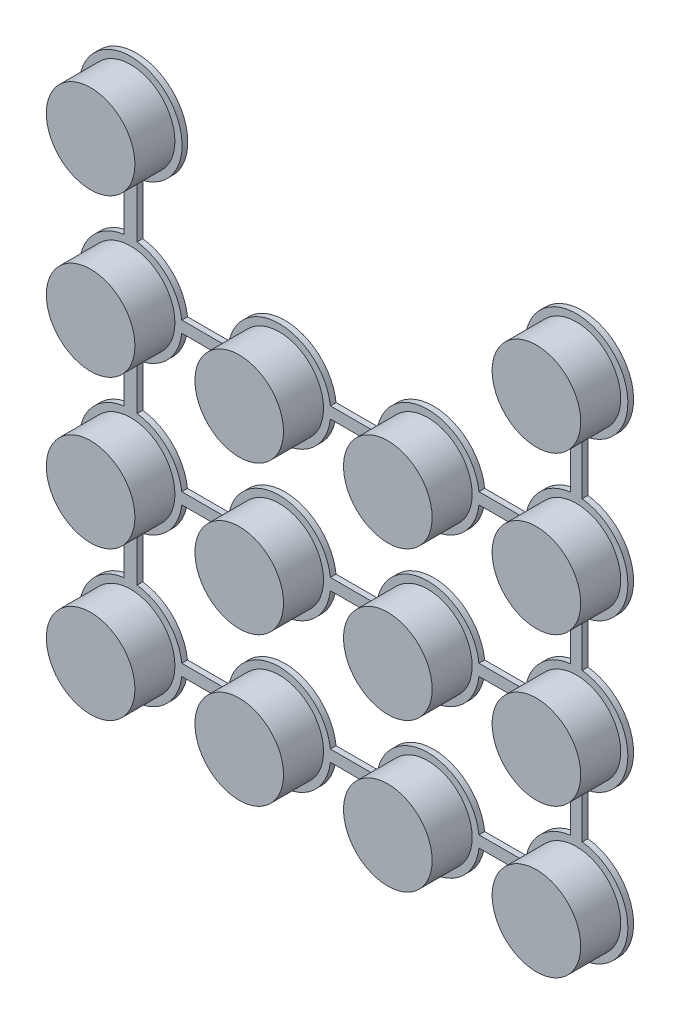
SolidWorks part; units mm, degrees
ref_plane "Front Plane" through (0, 0, 0) normal (0, 0, 1) x (1, 0, 0)
ref_plane "Top Plane" through (0, 0, 0) normal (0, 1, 0) x (1, 0, 0)
ref_plane "Right Plane" through (0, 0, 0) normal (1, 0, 0) x (0, 0, -1)
other "Configuration Table"
sketch "Sketch1" plane through (0, 0, 0) normal (0, 0, 1) x (1, 0, 0)
  line L0 (0, 0) -> (0, 200) construction
  line L9 (-37.875, 23) -> (-30, 23) construction
  line L10 (39, 48) -> (39, 58) construction
  line L15 (-37.875, 23) -> (-30, 23) construction
  line L16 (-40.125, 93.5706) -> (-40.125, 83.9294)
  line L17 (-37.875, 93.5706) -> (-37.875, 83.9294)
  line L18 (-30.0557, 76) -> (-21.9443, 76)
  line L19 (-30.0557, 74) -> (-21.9443, 74)
  line L20 (-30.0557, 50) -> (-21.9443, 50)
  line L21 (40, 23) -> (40, 102.5) construction
  line L22 (-30.0557, 48) -> (-21.9443, 48)
  line L23 (-30.0557, 22) -> (-21.9443, 22)
  line L24 (-30.0557, 24) -> (-21.9443, 24)
  line L25 (38, 31.9443) -> (38, 40.0557)
  line L26 (40, 31.9443) -> (40, 40.0557)
  line L27 (39, 23) -> (39, 102.5) construction
  line L28 (38, 23) -> (38, 102.5) construction
  line L29 (38, 83.9443) -> (38, 93.5557)
  line L30 (40, 83.9443) -> (40, 93.5557)
  line L31 (39, 74) -> (39, 76) construction
  line L32 (21.9443, 74) -> (30.0557, 74)
  line L33 (21.9443, 76) -> (30.0557, 76)
  line L35 (-5, 75) -> (0, 75) construction
  line L37 (-4.0557, 74) -> (4.0557, 74)
  line L39 (-4.0557, 76) -> (4.0557, 76)
  line L40 (-4.0557, 48) -> (4.0557, 48)
  line L44 (-4.0557, 50) -> (4.0557, 50)
  line L46 (-37.875, 66.0706) -> (-37.875, 57.9294)
  line L47 (-37.875, 40.0706) -> (-37.875, 31.9294)
  line L48 (-39, 22) -> (39, 22) construction
  line L50 (-40.125, 66.0706) -> (-40.125, 57.9294)
  line L51 (-40.125, 40.0706) -> (-40.125, 31.9294)
  line L52 (-39, 23) -> (39, 23) construction
  line L53 (-39, 24) -> (39, 24) construction
  line L55 (-4.0557, 24) -> (4.0557, 24)
  line L56 (-4.0557, 22) -> (4.0557, 22)
  line L57 (21.9443, 24) -> (30.0557, 24)
  line L58 (21.9443, 22) -> (30.0557, 22)
  line L59 (21.9443, 48) -> (30.0557, 48)
  line L60 (40, 57.9443) -> (40, 66.0557)
  line L61 (38, 57.9443) -> (38, 66.0557)
  line L62 (21.9443, 50) -> (30.0557, 50)
  arc A0 (-21.9443, 22) -> (-4.0557, 22) centre (-13, 23) ccw
  arc A1 (-40.125, 31.9294) -> (-30.0557, 22) centre (-39, 23) ccw
  arc A2 (-40.125, 57.9294) -> (-40.125, 40.0706) centre (-39, 49) ccw
  arc A3 (-4.0557, 50) -> (-21.9443, 50) centre (-13, 49) ccw
  arc A4 (-40.125, 83.9294) -> (-40.125, 66.0706) centre (-39, 75) ccw
  arc A5 (-4.0557, 76) -> (-21.9443, 76) centre (-13, 75) ccw
  arc A8 (-37.875, 93.5706) -> (-40.125, 93.5706) centre (-39, 102.5) ccw
  arc A10 (21.9443, 74) -> (4.0557, 74) centre (13, 75) cw
  arc A11 (40, 83.9443) -> (40, 66.0557) centre (39, 75) cw
  arc A12 (21.9443, 48) -> (4.0557, 48) centre (13, 49) cw
  arc A13 (38, 40.0557) -> (30.0557, 48) centre (39, 49) cw
  arc A14 (30.0557, 24) -> (38, 31.9443) centre (39, 23) cw
  arc A15 (4.0557, 24) -> (21.9443, 24) centre (13, 23) cw
  arc A16 (38, 93.5557) -> (40, 93.5557) centre (39, 102.5) cw
  arc A17 (30.0557, 76) -> (38, 83.9443) centre (39, 75) cw
  arc A18 (4.0557, 76) -> (21.9443, 76) centre (13, 75) cw
  arc A19 (-37.875, 66.0706) -> (-30.0557, 74) centre (-39, 75) ccw
  arc A20 (-37.875, 40.0706) -> (-30.0557, 48) centre (-39, 49) ccw
  arc A21 (-30.0557, 24) -> (-37.875, 31.9294) centre (-39, 23) ccw
  arc A22 (-4.0557, 24) -> (-21.9443, 24) centre (-13, 23) ccw
  arc A23 (21.9443, 22) -> (4.0557, 22) centre (13, 23) cw
  arc A24 (40, 31.9443) -> (30.0557, 22) centre (39, 23) cw
  arc A25 (30.0557, 50) -> (38, 57.9443) centre (39, 49) cw
  arc A26 (40, 57.9443) -> (40, 40.0557) centre (39, 49) cw
  arc A27 (38, 66.0557) -> (30.0557, 74) centre (39, 75) cw
  arc A28 (4.0557, 50) -> (21.9443, 50) centre (13, 49) cw
  arc A29 (-21.9443, 48) -> (-4.0557, 48) centre (-13, 49) ccw
  arc A30 (-30.0557, 50) -> (-37.875, 57.9294) centre (-39, 49) ccw
  arc A31 (-21.9443, 74) -> (-4.0557, 74) centre (-13, 75) ccw
  arc A32 (-30.0557, 76) -> (-37.875, 83.9294) centre (-39, 75) ccw
  point P11 (0, 151)
  dimension "D8" = 18
  dimension "D9" = 13
  dimension "D10" = 26
  dimension "D11" = 1
  dimension "D13" = 79.5
  dimension "D14" = 1
  dimension "D15" = 1
  dimension "D16" = 1
  dimension "D12" = 3
extrude "Boss-Extrude1" add sketch "Sketch1" along normal blind 1
sketch "Sketch2" plane through (0, 0, 1) normal (0, 0, 1) x (1, 0, 0)
  circle A0 centre (-39, 102.5) radius 7.75
  circle A1 centre (-39, 75) radius 7.75
  circle A2 centre (-39, 49) radius 7.75
  circle A3 centre (-39, 23) radius 7.75
  circle A4 centre (-13, 75) radius 7.75
  circle A6 centre (-13, 49) radius 7.75
  circle A7 centre (-13, 23) radius 7.75
  circle A8 centre (13, 75) radius 7.75
  circle A9 centre (39, 102.5) radius 7.75
  circle A10 centre (39, 23) radius 7.75
  circle A11 centre (13, 23) radius 7.75
  circle A12 centre (39, 49) radius 7.75
  circle A13 centre (13, 49) radius 7.75
  circle A14 centre (39, 75) radius 7.75
  dimension "D1" = 15.5
  dimension "D4" = 15.5
extrude "Boss-Extrude2" add sketch "Sketch2" along normal blind 7
